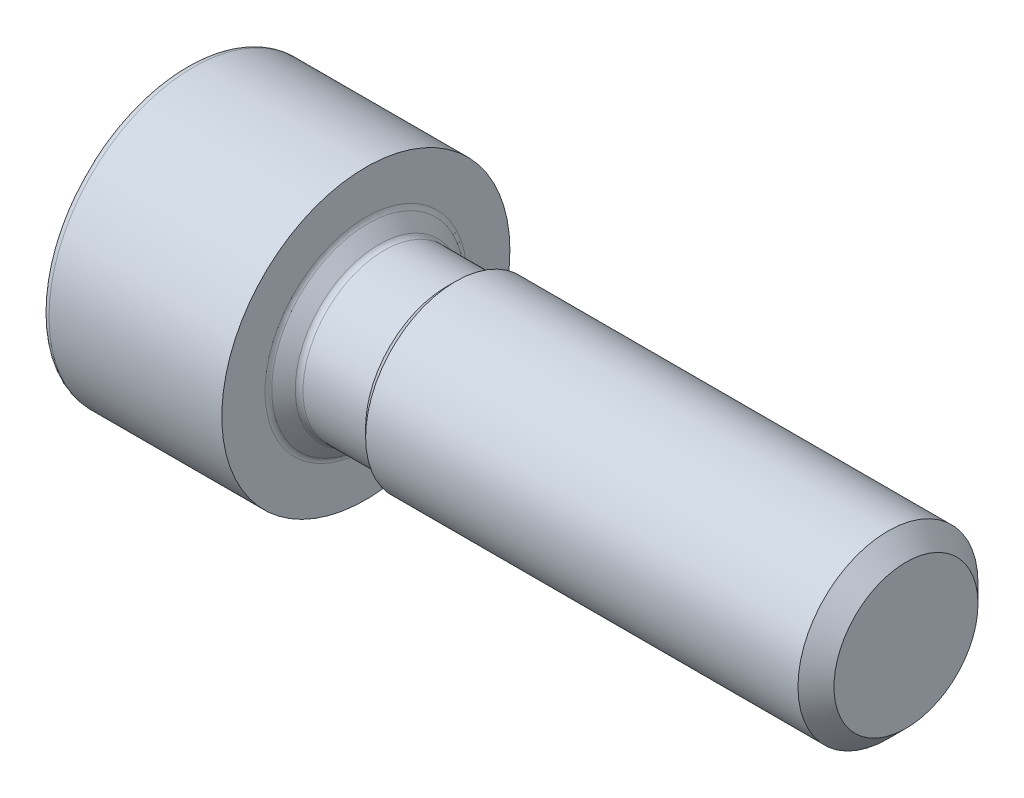
from build123d import *

# Parameters (mm, degrees)
CUT_EXTRUDE1_DEPTH = 6
FILLET1_R          = 0.4
CHAMFER1_SIZE      = 1


with BuildPart() as part:
    # Sketch1 → Base-Revolve (revolve)
    with BuildSketch(Plane.XY, mode=Mode.PRIVATE) as base_revolve_sk:
        with BuildLine():
            Line((0, 0), (0, 8))
            Line((0, 8), (10, 8))
            Line((10, 8), (10, 5.6))
            ThreePointArc((10, 5.6), (10.026649761, 5.456439562), (10.103047997, 5.332008381))
            Line((10.103047997, 5.332008381), (10.723047997, 4.645008381))
            ThreePointArc((10.723047997, 4.645008381), (10.857514074, 4.547488955), (11.02, 4.513))
            Line((11.02, 4.513), (14.5, 4.513))
            Line((14.5, 4.513), (14.987, 5))
            Line((14.987, 5), (40, 5))
            Line((40, 5), (40, 0))
            Line((40, 0), (0, 0))
        make_face()
    revolve(base_revolve_sk.sketch.rotate(Axis((0, 0, 0), (-1, 0, 0)), 90), axis=Axis((0, 0, 0), (-1, 0, 0)))

    # Sketch2 → Cut-Extrude1 (cut)
    with BuildSketch(Plane.ZY):
        Polygon((3.962066222, -2.2875), (3.962066222, 2.2875), (0, 4.575), (-3.962066222, 2.2875), (-3.962066222, -2.2875), (0, -4.575), align=None)
    extrude(amount=-CUT_EXTRUDE1_DEPTH, mode=Mode.SUBTRACT)

    # Sketch13 → Cut-Revolve4 (revolve, cut)
    with BuildSketch(Plane.XY):
        Polygon((0, 4.575), (0.612933778, 3.962066222), (0, 3.962066222), align=None)
    revolve(axis=Axis((0, 0, 0), (-1, 0, 0)), mode=Mode.SUBTRACT)

    # Sketch16 → Cut-Revolve5 (revolve, cut)
    with BuildSketch(Plane.XY, mode=Mode.PRIVATE) as cut_revolve5_sk:
        Polygon((8.641377482, 0), (6, 4.575), (6, 0), align=None)
    revolve(cut_revolve5_sk.sketch.rotate(Axis((6, 0, 0), (1, 0, 0)), 180), axis=Axis((6, 0, 0), (1, 0, 0)), mode=Mode.SUBTRACT)

    # Fillet1
    fillet1_edges = [part.edges().sort_by_distance(p)[0] for p in [
        (0, 0, 8),
    ]]
    fillet(fillet1_edges, radius=FILLET1_R)

    # Chamfer1
    chamfer1_edges = [part.edges().sort_by_distance(p)[0] for p in [
        (40, 0, 5),
    ]]
    chamfer(chamfer1_edges, length=CHAMFER1_SIZE)


solid = part.part
